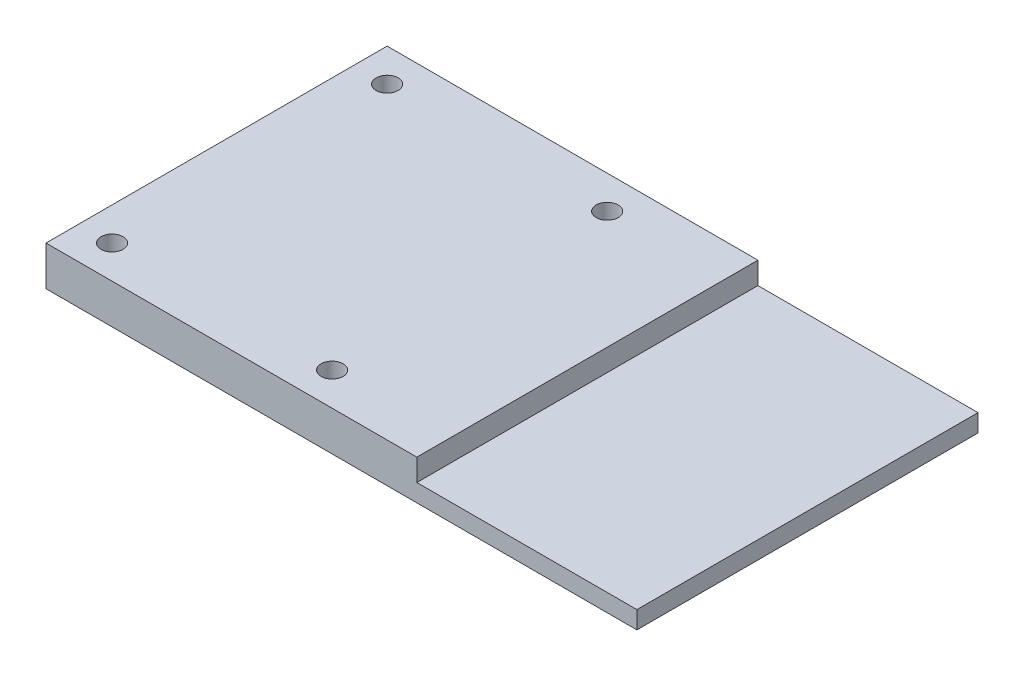
from build123d import *

# Parameters (mm, degrees)
SKETCH1_W           = 268.5
SKETCH1_H           = 155
BOSS_EXTRUDE1_DEPTH = 18
SKETCH2_R           = 5
CUT_EXTRUDE1_DEPTH  = 18
SKETCH3_W           = 100
SKETCH3_H           = 155
CUT_EXTRUDE2_DEPTH  = 10


with BuildPart() as part:
    # Sketch1 → Boss-Extrude1 (new body)
    with BuildSketch(Plane(origin=(0, 0, 0), x_dir=(1, 0, 0), z_dir=(0, 1, 0))):
        Rectangle(SKETCH1_W, SKETCH1_H)
    extrude(amount=BOSS_EXTRUDE1_DEPTH)

    # Sketch2 → Cut-Extrude1 (cut)
    with BuildSketch(Plane(origin=(0, 18, 0), x_dir=(1, 0, 0), z_dir=(0, 1, 0))):
        with Locations(Location((-119.25, 62.5, 0), (0, 0, 270))):
            Circle(SKETCH2_R)
        with Locations(Location((-19.25, 62.5, 0), (0, 0, 270))):
            Circle(SKETCH2_R)
        with Locations(Location((-19.25, -62.5, 0), (0, 0, 90))):
            Circle(SKETCH2_R)
        with Locations(Location((-119.25, -62.5, 0), (0, 0, 90))):
            Circle(SKETCH2_R)
    extrude(amount=-CUT_EXTRUDE1_DEPTH, mode=Mode.SUBTRACT)

    # Sketch3 → Cut-Extrude2 (cut)
    with BuildSketch(Plane(origin=(0, 18, 0), x_dir=(1, 0, 0), z_dir=(0, 1, 0))):
        with Locations((84.25, 0)):
            Rectangle(SKETCH3_W, SKETCH3_H)
    extrude(amount=-CUT_EXTRUDE2_DEPTH, mode=Mode.SUBTRACT)


solid = part.part
